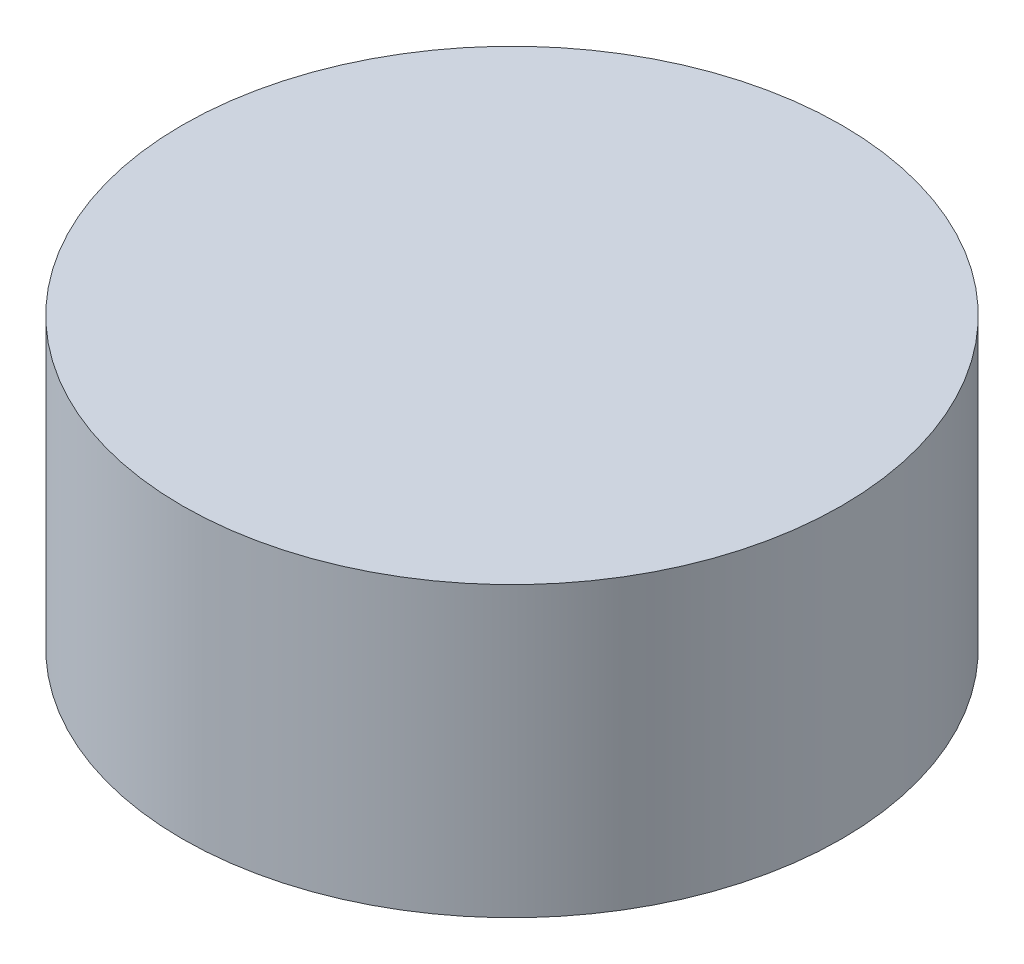
SolidWorks part; units mm, degrees
ref_plane "Front Plane" through (0, 0, 0) normal (0, 0, 1) x (1, 0, 0)
ref_plane "Top Plane" through (0, 0, 0) normal (0, 1, 0) x (1, 0, 0)
ref_plane "Right Plane" through (0, 0, 0) normal (1, 0, 0) x (0, 0, -1)
other "Configuration Table"
sketch "Sketch1" plane through (0, 0, 0) normal (0, 1, 0) x (1, 0, 0)
  circle A0 centre (0, 0) radius 16
  dimension "D1" = 32
extrude "Boss-Extrude1" add sketch "Sketch1" along normal blind 14
